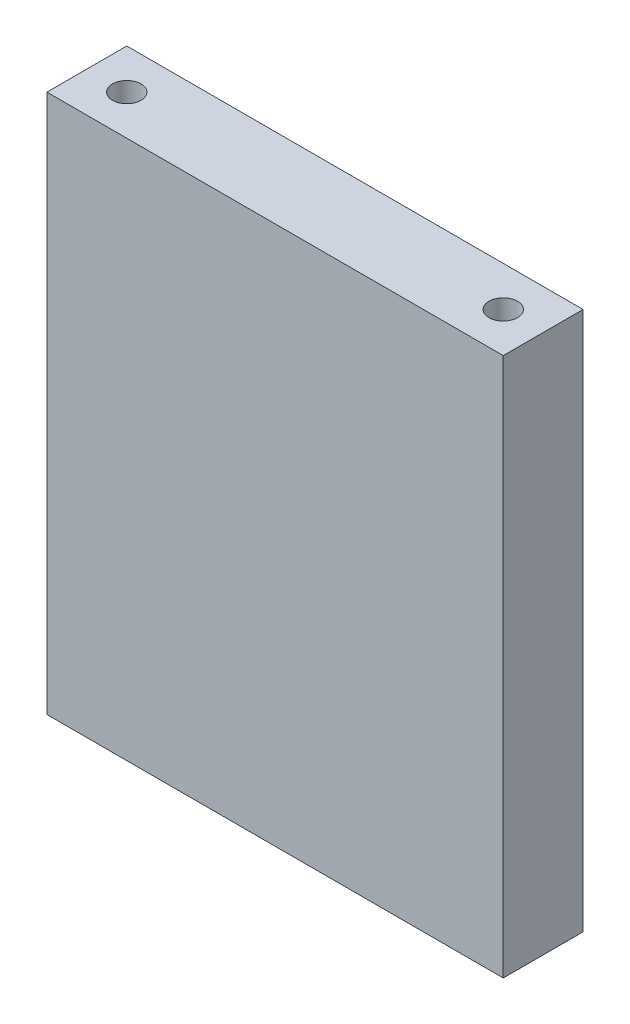
from build123d import *

# Parameters (mm, degrees)
SKETCH_1_W             = 80
SKETCH_1_H             = 94.5
EXTRUDE_1_DEPTH        = 14
HOLE_WIZARD_M6_1_D     = 5
HOLE_WIZARD_M6_1_DEPTH = 17
HOLE_WIZARD_M6_1_TIP   = 1.502151548
HOLE_WIZARD_M6_2_D     = 5
HOLE_WIZARD_M6_2_DEPTH = 17
HOLE_WIZARD_M6_2_TIP   = 1.502151548


with BuildPart() as part:
    # 草图1 → 凸台-拉伸1 (new body)
    with BuildSketch(Plane.XY):
        Rectangle(SKETCH_1_W, SKETCH_1_H)
    extrude(amount=EXTRUDE_1_DEPTH)

    # M6 螺纹孔1
    with Locations(Plane(origin=(0, -47.25, 0), x_dir=(-1, 0, 0), z_dir=(0, -1, 0))):
        with Locations((-21, -7), (21, -7)):
            Hole(HOLE_WIZARD_M6_1_D / 2, depth=HOLE_WIZARD_M6_1_DEPTH)
            with Locations((0, 0, -(HOLE_WIZARD_M6_1_DEPTH + HOLE_WIZARD_M6_1_TIP / 2))):  # 118° drill point
                Cone(0, HOLE_WIZARD_M6_1_D / 2, HOLE_WIZARD_M6_1_TIP, mode=Mode.SUBTRACT)

    # M6 螺纹孔2
    with Locations(Plane(origin=(0, 47.25, 0), x_dir=(1, 0, 0), z_dir=(0, 1, 0))):
        with Locations((33, -7), (-33, -7)):
            Hole(HOLE_WIZARD_M6_2_D / 2, depth=HOLE_WIZARD_M6_2_DEPTH)
            with Locations((0, 0, -(HOLE_WIZARD_M6_2_DEPTH + HOLE_WIZARD_M6_2_TIP / 2))):  # 118° drill point
                Cone(0, HOLE_WIZARD_M6_2_D / 2, HOLE_WIZARD_M6_2_TIP, mode=Mode.SUBTRACT)


solid = part.part
